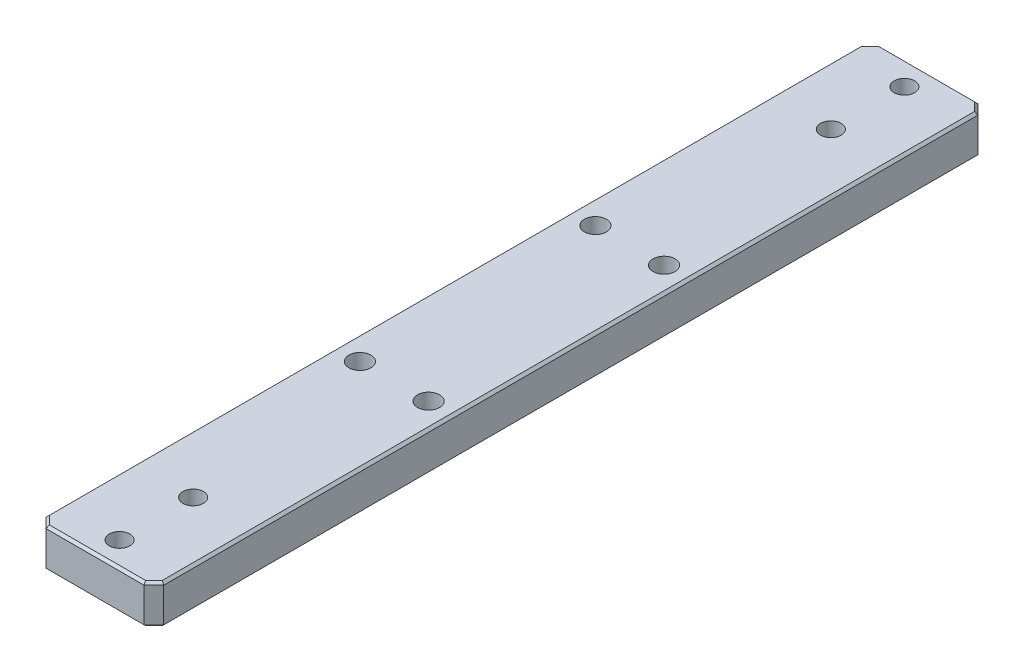
SolidWorks part; units mm, degrees
material "Al6061"
ref_plane "Front" through (0, 0, 0) normal (0, 0, 1) x (1, 0, 0)
ref_plane "Top" through (0, 0, 0) normal (0, 1, 0) x (1, 0, 0)
ref_plane "Right" through (0, 0, 0) normal (1, 0, 0) x (0, 0, -1)
sketch "草图1" plane through (0, 0, 0) normal (0, 1, 0) x (1, 0, 0)
  line L1 (-12, 85) -> (12, 85)
  line L2 (-12, 85) -> (-12, -85)
  line L3 (-12, -85) -> (12, -85)
  line L4 (12, 85) -> (12, -85)
  line L5 (-12, 85) -> (12, -85) construction
  line L6 (-12, -85) -> (12, 85) construction
  point P0 (0, 0)
  dimension "D1" = 170
  dimension "D2" = 24
extrude "凸台-拉伸1" add sketch "草图1" along normal blind 8
hole_wizard "M4 六角凹头螺钉的柱形沉头孔1" positions "草图3" profile "草图2" counterbore size "M4" standard "Iso" end condition through all
sketch "草图3" plane through (0, 0, 0) normal (0, -1, 0) x (-1, 0, 0)
  line L0 (-7, 24) -> (-7, -24) construction
  line L2 (0, 0) -> (-7, 0) construction
  line L4 (12, 85) -> (12, -85) construction
  point P0 (-7, 24)
  point P2 (7, 24)
  point P4 (-7, -24)
  point P6 (7, -24)
  dimension "D1" = 5
  dimension "D2" = 14
  dimension "D3" = 48
sketch "草图2" plane through (7, 0, -24) normal (1, 0, 0) x (0, 0, -1)
  line L0 (0, 0) -> (0, 8)
  line L1 (0, 8) -> (2.25, 8)
  line L3 (2.25, 8) -> (2.25, 4.4)
  line L4 (2.25, 4.4) -> (4, 4.4)
  line L5 (4, 4.4) -> (4, 0)
  line L7 (4, 0) -> (0, 0)
  line L11 (0, -6.35) -> (0, 107.95) construction
  dimension "通孔孔直径" = 4.5
  dimension "通孔孔深度" = 8
  dimension "柱形沉头孔直径" = 8
  dimension "柱形沉头孔深度" = 4.4
hole_wizard "M5 螺纹孔1" positions "草图5" profile "草图4" tap size "M5" standard "Iso"
sketch "草图5" plane through (0, 8, 0) normal (0, 1, 0) x (1, 0, 0)
  line L0 (0, 80) -> (0, -80) construction
  point P0 (0, 80)
  point P2 (0, -80)
  point P19 (0, -65)
  point P21 (0, 65)
  dimension "D1" = 15
  dimension "D2" = 160
  dimension "D3" = 15
sketch "草图4" plane through (0, 8, -80) normal (1, 0, 0) x (0, 0, 1)
  line L0 (0, 0) -> (0, 13.6618)
  line L1 (0, 13.6618) -> (2.1, 12.4)
  line L2 (2.1, 12.4) -> (2.1, 0)
  line L5 (2.1, 0) -> (0, 0)
  line L10 (0, 13.6618) -> (-2.1, 12.4) construction
  line L11 (0, -6.35) -> (0, 107.95) construction
  dimension "螺纹孔钻头直径" = 4.2
  dimension "螺纹孔钻头深度" = 12.4
  dimension "导头角度" = 118
cosmetic thread "孔螺蚊线1" parameters "D1"=8, "D2"=5
cosmetic thread "孔螺蚊线2" parameters "D1"=8, "D2"=5
cosmetic thread "孔螺蚊线3" parameters "D1"=8, "D2"=5
cosmetic thread "孔螺蚊线4" parameters "D1"=8, "D2"=5
chamfer "倒角1" distance 2 angle 45 4 edges at (-12, 4, -85) (12, 4, -85) (-12, 4, 85) (12, 4, 85)
chamfer "倒角2" distance 0.5 angle 45 16 edges at (11, 0, -84) (0, 0, -85) (-11, 0, -84) (-12, 0, 0) (-11, 0, 84) (0, 0, 85) (12, 0, 0) (11, 0, 84) (11, 8, 84) (0, 8, 85) (-11, 8, 84) (-12, 8, 0) (-11, 8, -84) (0, 8, -85) (11, 8, -84) (12, 8, 0)
